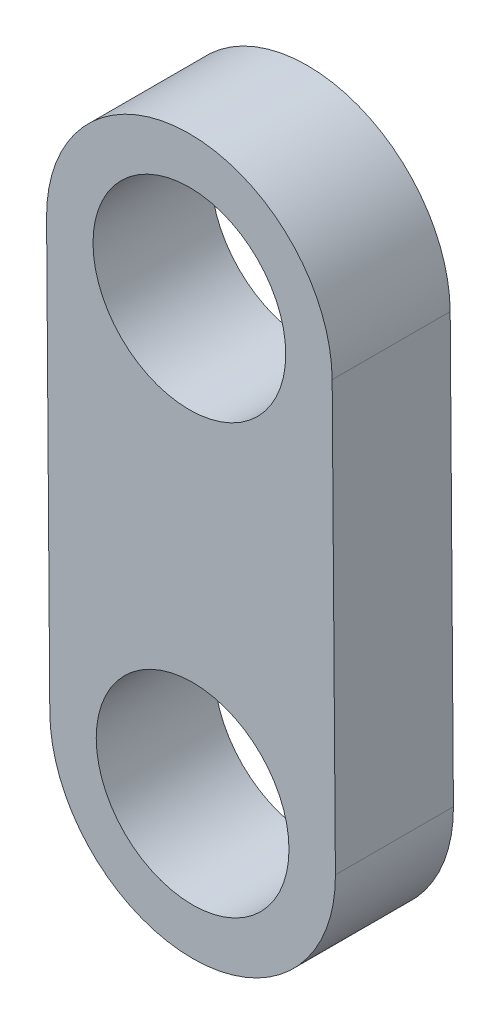
SolidWorks part; units mm, degrees
ref_plane "Front Plane" through (0, 0, 0) normal (0, 0, 1) x (1, 0, 0)
ref_plane "Top Plane" through (0, 0, 0) normal (0, 1, 0) x (1, 0, 0)
ref_plane "Right Plane" through (0, 0, 0) normal (1, 0, 0) x (0, 0, -1)
other "Configuration Table"
sketch "Sketch1" plane through (0, 0, 0) normal (0, 0, 1) x (1, 0, 0)
  line L2 (31.6962, -16.2201) -> (31.573, 0.0682)
  line L3 (20.6834, -0.0142) -> (20.8066, -16.3025)
  circle A1 centre (26.1282, 0.027) radius 3.6746
  arc A5 (31.573, 0.0682) -> (20.6834, -0.0142) centre (26.1282, 0.027) ccw
  arc A6 (20.8066, -16.3025) -> (31.6962, -16.2201) centre (26.2514, -16.2613) ccw
  circle A9 centre (26.2514, -16.2613) radius 3.6746
extrude "Boss-Extrude1" add sketch "Sketch1" along normal up to surface (4.5 mm away)
